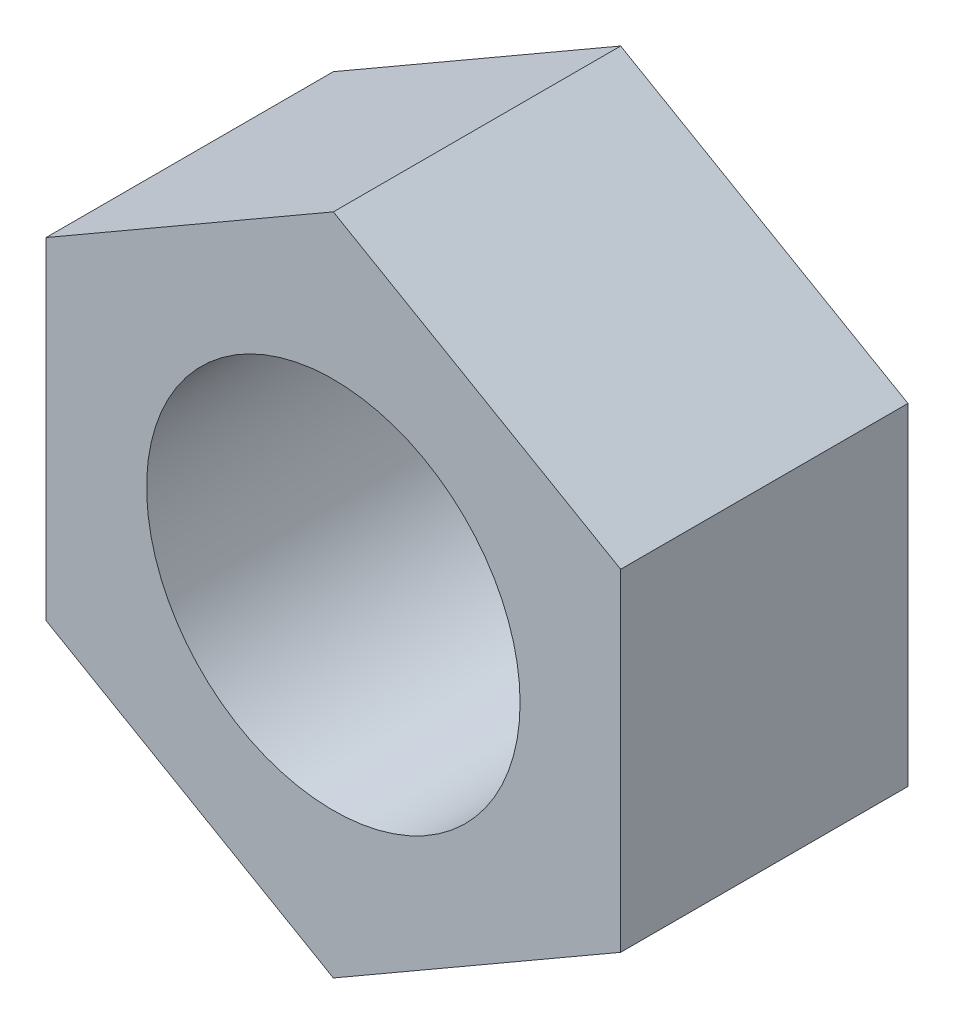
from build123d import *

# Parameters (mm, degrees)
SKETCH1_R           = 5.2
BOSS_EXTRUDE1_DEPTH = 8


with BuildPart() as part:
    # Sketch1 → Boss-Extrude1 (new body)
    with BuildSketch(Plane.XY):
        Polygon((0, 9.237604307), (-8, 4.618802154), (-8, -4.618802154), (0, -9.237604307), (8, -4.618802154), (8, 4.618802154), align=None)
        Circle(SKETCH1_R, mode=Mode.SUBTRACT)
    extrude(amount=BOSS_EXTRUDE1_DEPTH)


solid = part.part
